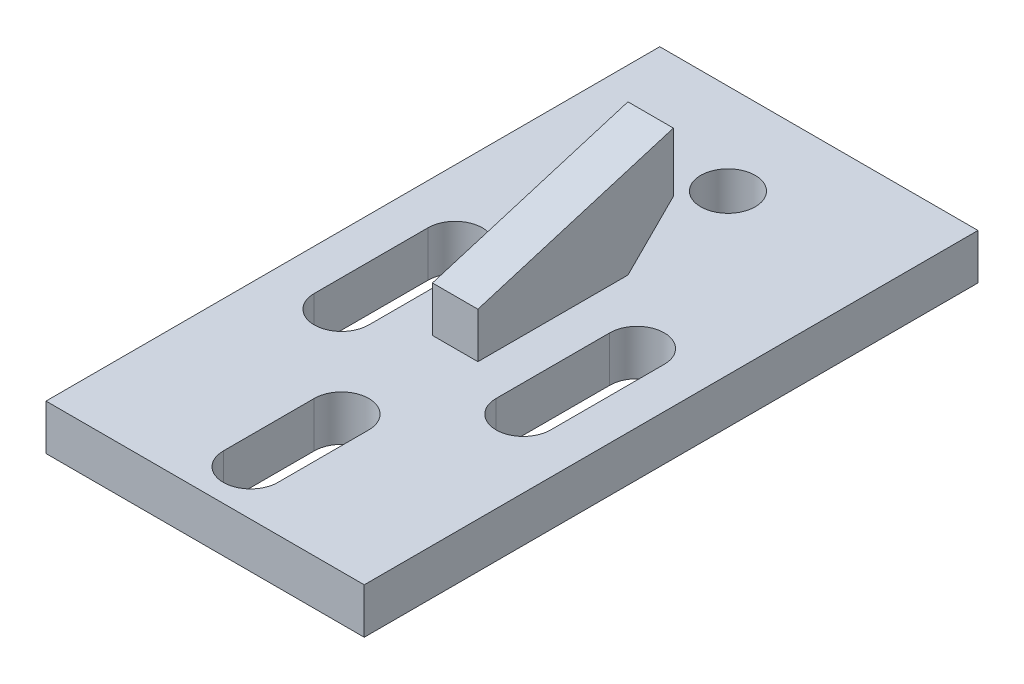
SolidWorks part; units mm, degrees
material "A3"
ref_plane "前视基准面" through (0, 0, 0) normal (0, 0, 1) x (1, 0, 0)
ref_plane "上视基准面" through (0, 0, 0) normal (0, 1, 0) x (1, 0, 0)
ref_plane "右视基准面" through (0, 0, 0) normal (1, 0, 0) x (0, 0, -1)
sketch "草图1" plane through (0, 0, 0) normal (0, 1, 0) x (1, 0, 0)
  line L0 (0, 47.5) -> (0, -67.5) construction
  line L1 (-35, -67.5) -> (35, -67.5)
  line L2 (-35, -67.5) -> (-35, 67.5)
  line L3 (-35, 67.5) -> (35, 67.5)
  line L4 (35, -67.5) -> (35, 67.5)
  line L5 (-35, -67.5) -> (35, 67.5) construction
  line L6 (-35, 67.5) -> (35, -67.5) construction
  line L7 (0, -37.5) -> (0, -57.5) construction
  line L8 (6, -37.5) -> (6, -57.5)
  line L9 (-6, -37.5) -> (-6, -57.5)
  line L10 (-20, 7.5) -> (-20, -17.5) construction
  line L11 (-14, 7.5) -> (-14, -17.5)
  line L12 (-26, 7.5) -> (-26, -17.5)
  line L13 (20, 7.5) -> (20, -17.5) construction
  line L14 (14, 7.5) -> (14, -17.5)
  line L15 (26, 7.5) -> (26, -17.5)
  circle A0 centre (0, 47.5) radius 6
  arc A1 (6, -37.5) -> (-6, -37.5) centre (0, -37.5) ccw
  arc A2 (-6, -57.5) -> (6, -57.5) centre (0, -57.5) ccw
  arc A3 (-14, 7.5) -> (-26, 7.5) centre (-20, 7.5) ccw
  arc A4 (-26, -17.5) -> (-14, -17.5) centre (-20, -17.5) ccw
  arc A5 (14, 7.5) -> (26, 7.5) centre (20, 7.5) cw
  arc A6 (26, -17.5) -> (14, -17.5) centre (20, -17.5) cw
  point P0 (0, 0)
  point P11 (0, -47.5)
  point P16 (-20, -5)
  point P25 (20, -5)
  dimension "D3" = 12
  dimension "D5" = 6
  dimension "D8" = 6
  dimension "D9" = 40
  dimension "D1" = 135
  dimension "D2" = 70
  dimension "D4" = 115
  dimension "D6" = 20
  dimension "D7" = 25
  dimension "D10" = 20
  dimension "D11" = 45
extrude "凸台-拉伸1" add sketch "草图1" along normal blind 10
sketch "草图2" plane through (0, 0, 0) normal (1, 0, 0) x (0, 0, -1)
  line L0 (-12.5, 10) -> (-12.5, 20)
  line L1 (-67.5, 10) -> (67.5, 10) construction
  line L2 (-12.5, 20) -> (30.5, 33)
  line L3 (30.5, 33) -> (30.5, 20)
  line L4 (30.5, 20) -> (20.5, 10)
  line L5 (20.5, 10) -> (-12.5, 10)
  line L6 (-67.5, 10) -> (-67.5, 0) construction
  dimension "D1" = 10
  dimension "D2" = 43
  dimension "D3" = 23
  dimension "D4" = 45
  dimension "D5" = 98
  dimension "D6" = 10
extrude "凸台-拉伸2" add sketch "草图2" along normal mid plane 10 separate body
